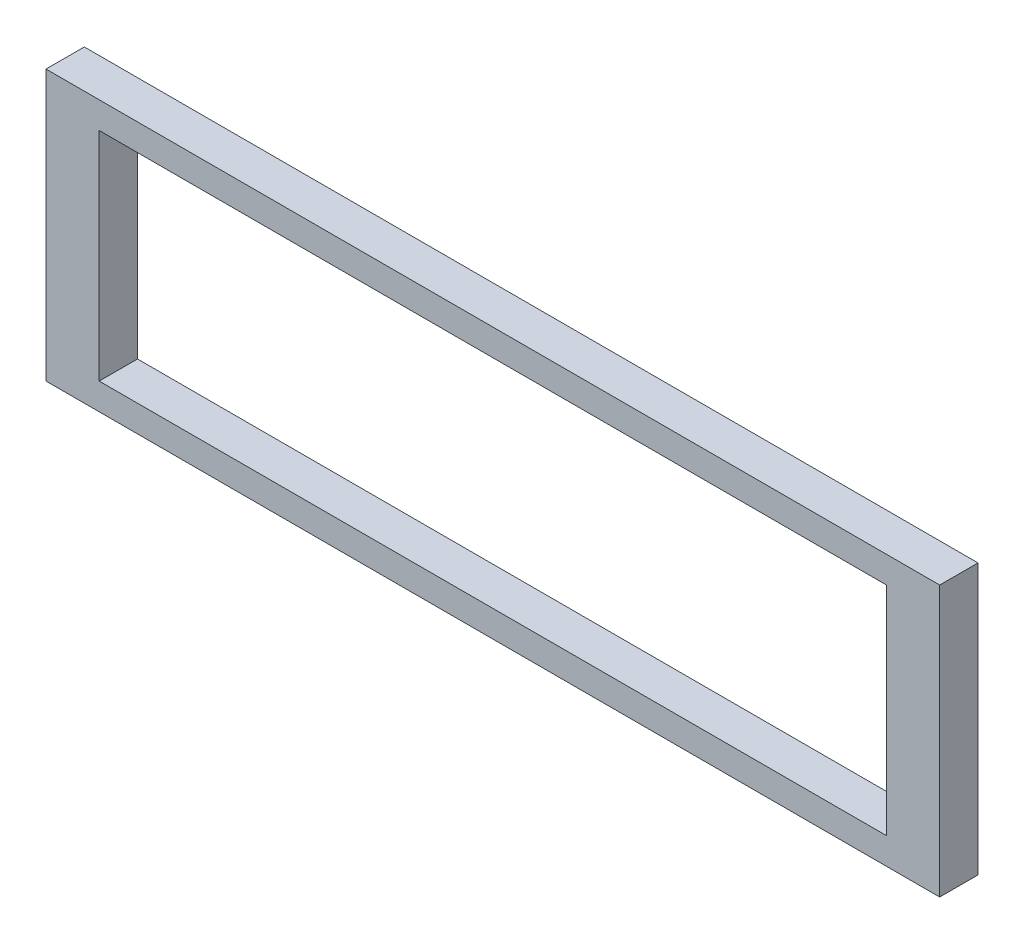
SolidWorks part; units mm, degrees
ref_plane "前视基准面" through (0, 0, 0) normal (0, 0, 1) x (1, 0, 0)
ref_plane "上视基准面" through (0, 0, 0) normal (0, 1, 0) x (1, 0, 0)
ref_plane "右视基准面" through (0, 0, 0) normal (1, 0, 0) x (0, 0, -1)
other "Configuration Table"
sketch "草图1" plane through (0, 0, 0) normal (0, 0, 1) x (1, 0, 0)
  line L0 (-210, -63.5) -> (210, -63.5)
  line L1 (210, -63.5) -> (210, 63.5)
  line L2 (210, 63.5) -> (-210, 63.5)
  line L3 (-210, 63.5) -> (-210, -63.5)
  line L4 (-185, -51) -> (185, -51)
  line L5 (185, -51) -> (185, 51)
  line L6 (185, 51) -> (-185, 51)
  line L7 (-185, 51) -> (-185, -51)
  point P0 (0, 0)
  dimension "D1" = 25
  dimension "D2" = 210
  dimension "D3" = 395
  dimension "D4" = 420
  dimension "D5" = 12.5
  dimension "D6" = 63.5
  dimension "D7" = 114.5
  dimension "D8" = 127
extrude "凸台-拉伸1" add sketch "草图1" against normal mid plane 18
